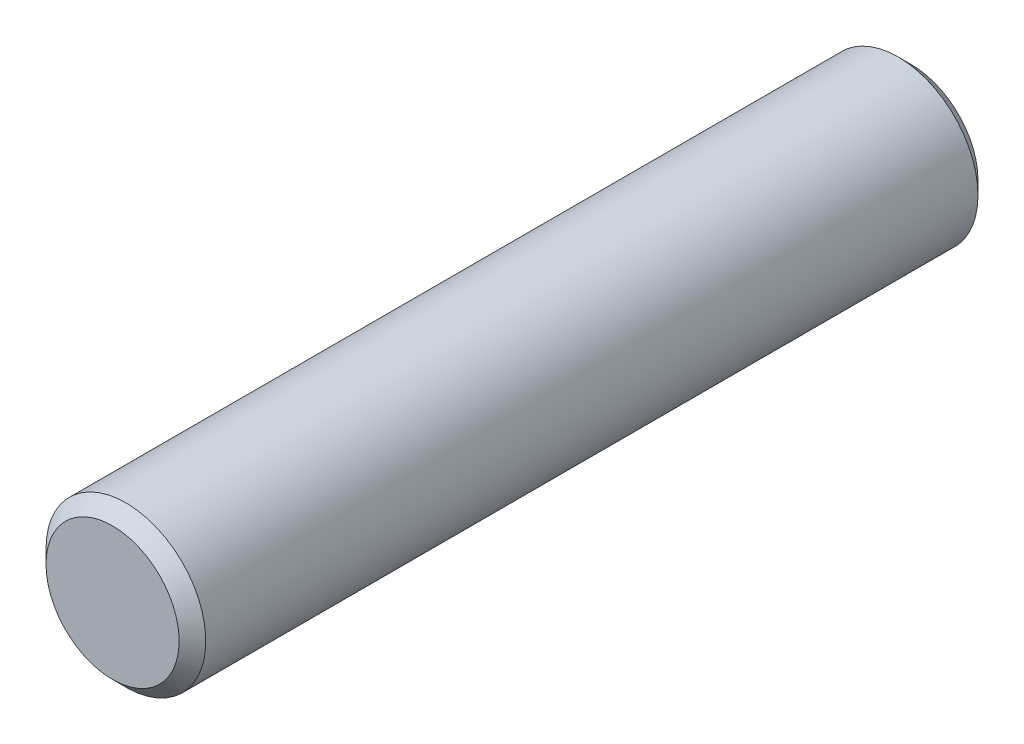
SolidWorks part; units mm, degrees
ref_plane "Front Plane" through (0, 0, 0) normal (0, 0, 1) x (1, 0, 0)
ref_plane "Top Plane" through (0, 0, 0) normal (0, 1, 0) x (1, 0, 0)
ref_plane "Right Plane" through (0, 0, 0) normal (1, 0, 0) x (0, 0, -1)
sketch "Sketch1" plane through (0, 0, 0) normal (0, 0, 1) x (1, 0, 0)
  circle A0 centre (0, 0) radius 3
  dimension "D1" = 6
extrude "Boss-Extrude1" add sketch "Sketch1" along normal blind 30
chamfer "Chamfer1" distance 0.5 angle 45 2 edges at (3, 0, 0) (3, 0, 30)
